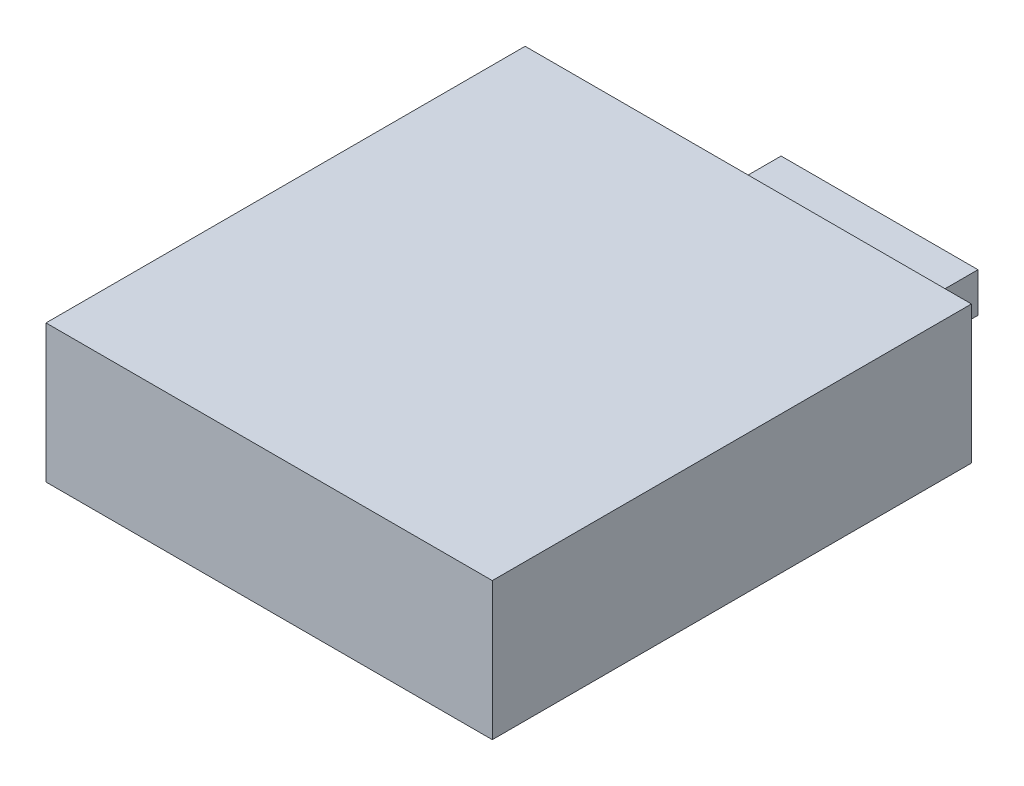
from build123d import *

# Parameters (mm, degrees)
SKETCH1_W           = 68
SKETCH1_H           = 73
BOSS_EXTRUDE1_DEPTH = 21
SKETCH2_W           = 30
SKETCH2_H           = 6.020166846
BOSS_EXTRUDE2_DEPTH = 20
SKETCH3_R           = 3
CUT_EXTRUDE1_DEPTH  = 20


with BuildPart() as part:
    # Sketch1 → Boss-Extrude1 (new body)
    with BuildSketch(Plane(origin=(0, 0, 0), x_dir=(1, 0, 0), z_dir=(0, 1, 0))):
        Rectangle(SKETCH1_W, SKETCH1_H)
    extrude(amount=BOSS_EXTRUDE1_DEPTH)

    # Sketch2 → Boss-Extrude2 (add)
    with BuildSketch(Plane(origin=(0, 0, -36.5), x_dir=(-1, 0, 0), z_dir=(0, 0, -1))):
        with Locations((0, 3.010083423)):
            Rectangle(SKETCH2_W, SKETCH2_H)
    extrude(amount=BOSS_EXTRUDE2_DEPTH)

    # Sketch3 → Cut-Extrude1 (cut)
    with BuildSketch(Plane(origin=(0, 6.020166846, 0), x_dir=(1, 0, 0), z_dir=(0, 1, 0))):
        with Locations(Location((9.5, 48.256848867, 0), (0, 0, 180))):
            Circle(SKETCH3_R)
        with Locations(Location((-9.5, 48.256848867, 0), (0, 0, 180))):
            Circle(SKETCH3_R)
    extrude(amount=-CUT_EXTRUDE1_DEPTH, mode=Mode.SUBTRACT)


solid = part.part
